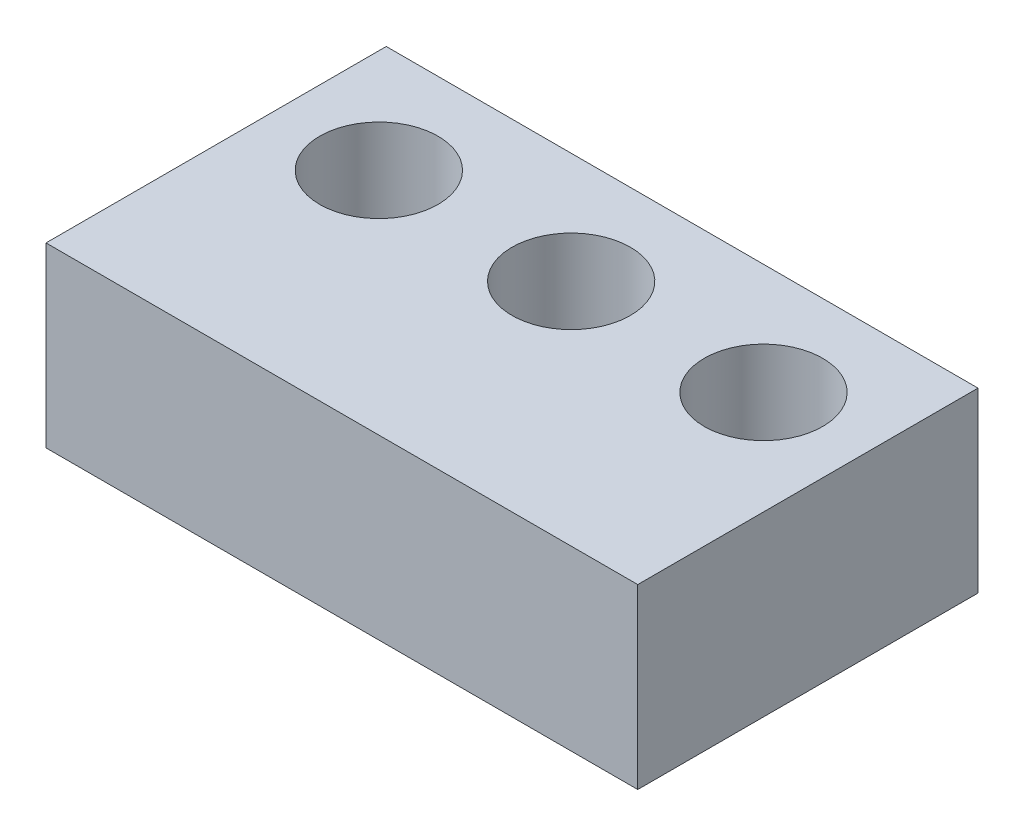
from build123d import *

# Parameters (mm, degrees)
SKETCH_1_W          = 40
SKETCH_1_H          = 12
EXTRUDE_1_DEPTH     = 7.5
CUT_EXTRUDE_1_REACH = 26.5
SKETCH_2_R          = 4
CUT_EXTRUDE_2_REACH = 26.5
SKETCH_3_R          = 4
SKETCH_6_W          = 40
SKETCH_6_H          = 12
EXTRUDE_3_DEPTH     = 8


with BuildPart() as part:
    # 草图1 → 凸台-拉伸1 (new, symmetric)
    with BuildSketch(Plane.XY):
        Rectangle(SKETCH_1_W, SKETCH_1_H)
    extrude(amount=EXTRUDE_1_DEPTH, both=True)

    # 草图2 → 切除-拉伸1 (cut, up to next)
    with BuildSketch(Plane(origin=(0, 6, 0), x_dir=(1, 0, 0), z_dir=(0, 1, 0)), mode=Mode.PRIVATE) as cut_extrude_1_sk1:
        with Locations(Location((-13, 0, 0), (0, 0, 270))):
            Circle(SKETCH_2_R)
    cut_extrude_1_tool1 = extrude(cut_extrude_1_sk1.sketch, amount=-CUT_EXTRUDE_1_REACH, mode=Mode.PRIVATE) & part.part
    # 草图2 → 切除-拉伸1 (cut, up to next)
    with BuildSketch(Plane(origin=(0, 6, 0), x_dir=(1, 0, 0), z_dir=(0, 1, 0)), mode=Mode.PRIVATE) as cut_extrude_1_sk2:
        with Locations(Location((13, 0, 0), (0, 0, 270))):
            Circle(SKETCH_2_R)
    cut_extrude_1_tool2 = extrude(cut_extrude_1_sk2.sketch, amount=-CUT_EXTRUDE_1_REACH, mode=Mode.PRIVATE) & part.part
    add(cut_extrude_1_tool1.solids().sort_by_distance((-13, 6, 0))[0], mode=Mode.SUBTRACT)
    add(cut_extrude_1_tool2.solids().sort_by_distance((13, 6, 0))[0], mode=Mode.SUBTRACT)

    # 草图3 → 切除-拉伸2 (cut, up to next)
    with BuildSketch(Plane.XZ.offset(6), mode=Mode.PRIVATE) as cut_extrude_2_sk1:
        with Locations(Location((0, 0, 0), (0, 0, 270))):
            Circle(SKETCH_3_R)
    cut_extrude_2_tool1 = extrude(cut_extrude_2_sk1.sketch, amount=-CUT_EXTRUDE_2_REACH, mode=Mode.PRIVATE) & part.part
    add(cut_extrude_2_tool1.solids().sort_by_distance((0, -6, 0))[0], mode=Mode.SUBTRACT)

    # 草图6 → 凸台-拉伸3 (add)
    with BuildSketch(Plane.XY.offset(7.5)):
        Rectangle(SKETCH_6_W, SKETCH_6_H)
    extrude(amount=EXTRUDE_3_DEPTH)


solid = part.part
